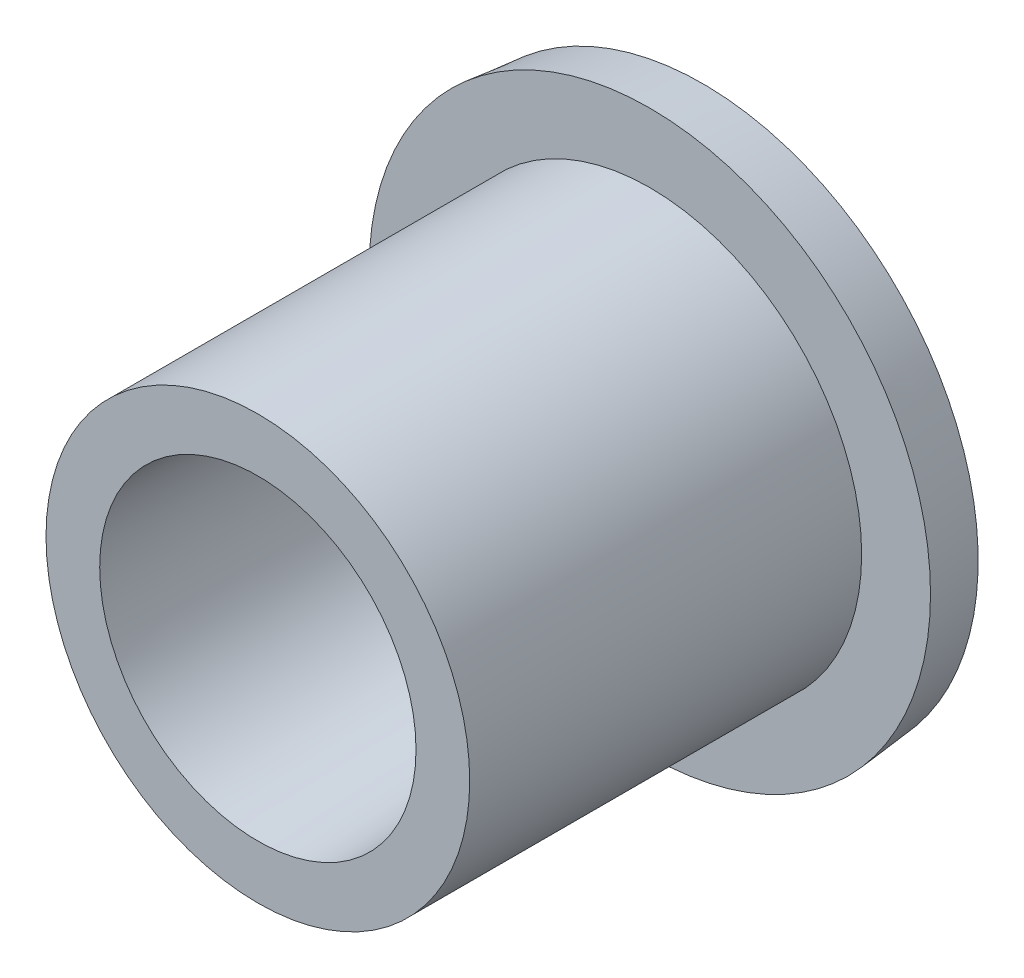
SolidWorks part; units mm, degrees
ref_plane "Front Plane" through (0, 0, 0) normal (0, 0, 1) x (1, 0, 0)
ref_plane "Top Plane" through (0, 0, 0) normal (0, 1, 0) x (1, 0, 0)
ref_plane "Right Plane" through (0, 0, 0) normal (1, 0, 0) x (0, 0, -1)
other "Configuration Table"
sketch "Sketch1" plane through (0, 318.5, 0) normal (0, -1, 0) x (-1, 0, 0)
  line L0 (0, 174.5) -> (0, 26.1) construction
  line L1 (40, 164.5) -> (40, 90.5)
  line L2 (26, 174.5) -> (52, 174.5)
  line L3 (52, 174.5) -> (53, 164.5)
  line L4 (53, 164.5) -> (40, 164.5)
  line L5 (40, 90.5) -> (29.8621, 90.5)
  line L17 (222, 50.1) -> (219, 50.1)
  line L18 (222, 53.1) -> (222, 50.1)
  line L19 (227, 53.1) -> (222, 53.1)
  line L20 (227, 26.1) -> (227, 53.1)
  line L21 (0, 26.1) -> (227, 26.1)
  line L22 (0, 174.5) -> (0, 26.1)
  line L23 (26, 174.5) -> (0, 174.5)
  line L24 (30, 87.5) -> (26, 174.5)
  line L25 (176, 87.5) -> (30, 87.5)
  line L26 (176, 77.5) -> (176, 87.5)
  line L27 (196, 77.5) -> (176, 77.5)
  line L28 (196, 51.1) -> (196, 77.5)
  line L29 (196, 50.1) -> (196, 51.1)
  line L30 (199, 50.1) -> (196, 50.1)
  line L31 (199, 51.1) -> (199, 50.1)
  line L32 (219, 51.1) -> (199, 51.1)
  line L33 (219, 50.1) -> (219, 51.1)
  line L34 (222, 50.1) -> (219, 50.1) construction
  line L35 (222, 53.1) -> (222, 50.1) construction
  line L36 (227, 53.1) -> (222, 53.1) construction
  line L37 (227, 26.1) -> (227, 53.1) construction
  line L38 (0, 26.1) -> (227, 26.1) construction
  line L40 (26, 174.5) -> (0, 174.5) construction
  line L41 (29.8621, 90.5) -> (26, 174.5)
  line L42 (176, 87.5) -> (30, 87.5) construction
  line L43 (176, 77.5) -> (176, 87.5) construction
  line L44 (196, 77.5) -> (176, 77.5) construction
  line L45 (196, 51.1) -> (196, 77.5) construction
  line L46 (196, 50.1) -> (196, 51.1) construction
  line L47 (199, 50.1) -> (196, 50.1) construction
  line L48 (199, 51.1) -> (199, 50.1) construction
  line L49 (219, 51.1) -> (199, 51.1) construction
  line L50 (219, 50.1) -> (219, 51.1) construction
  dimension "D2" = 84
  dimension "D3" = 40
  dimension "D4" = 52
  dimension "D5" = 53
  dimension "D6" = 10
  dimension "D1" = 0
revolve "Revolve1" add sketch "Sketch1" angle 360 about L0
